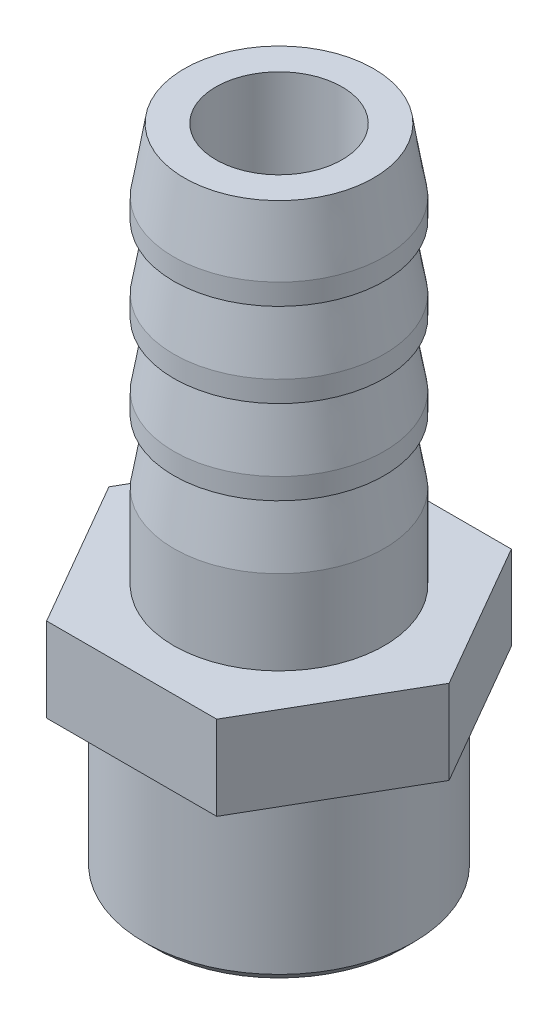
SolidWorks part; units mm, degrees
ref_plane "前视基准面" through (0, 0, 0) normal (0, 0, 1) x (1, 0, 0)
ref_plane "上视基准面" through (0, 0, 0) normal (0, 1, 0) x (1, 0, 0)
ref_plane "右视基准面" through (0, 0, 0) normal (1, 0, 0) x (0, 0, -1)
sketch "草图1" plane through (0, 0, 0) normal (0, 0, 1) x (1, 0, 0)
  line L0 (0, -266.5887) -> (0, 13062.8486) construction
  line L1 (-5, 4) -> (-4.5, 7)
  line L2 (0, 0) -> (-5, 0)
  line L3 (0, 0) -> (0, 19)
  line L5 (-5, 0) -> (-5, 4)
  line L6 (-5, 8) -> (-4.5, 11)
  line L7 (-5, 7) -> (-4.5, 7)
  line L8 (-5, 7) -> (-5, 8)
  line L11 (-4.5, -988.826) -> (-4.5, 49011.174) construction
  line L12 (-5, 11) -> (-4.5, 11)
  line L13 (-5, 11) -> (-5, 12)
  line L16 (-5, 12) -> (-4.5, 15)
  line L17 (-5, 15) -> (-4.5, 15)
  line L18 (-5, 15) -> (-5, 16)
  line L19 (-5, 16) -> (-4.5, 19)
  line L20 (-4.5, 19) -> (0, 19)
  point P9 (-5, 0.826)
  dimension "D1" = 5
  dimension "D2" = 19
  dimension "D3" = 1
  dimension "D4" = 3
  dimension "D5" = 4.5
  dimension "D6" = 1
  dimension "D7" = 3
  dimension "D8" = 3
  dimension "D9" = 1
  dimension "D10" = 3
revolve "旋转1" add sketch "草图1" angle 360 about L3
sketch "草图2" plane through (0, 0, 0) normal (0, -1, 0) x (1, 0, 0)
  line L0 (-1000, 0) -> (49000, 0) construction
  line L1 (8.0829, 0) -> (4.0415, 7)
  line L2 (4.0415, 7) -> (-4.0415, 7)
  line L3 (-4.0415, 7) -> (-8.0829, 0)
  line L4 (-8.0829, 0) -> (-4.0415, -7)
  line L5 (-4.0415, -7) -> (4.0415, -7)
  line L6 (4.0415, -7) -> (8.0829, 0)
  circle A0 centre (0, 0) radius 7 construction
  dimension "D1" = 14
extrude "凸台-拉伸1" add sketch "草图2" along normal blind 4
sketch "草图3" plane through (0, -4, 0) normal (0, -1, 0) x (1, 0, 0)
  circle A0 centre (0, 0) radius 6.4
  dimension "D1" = 12.8
extrude "凸台-拉伸2" add sketch "草图3" along normal blind 8
cosmetic thread "装饰螺纹线1" parameters "D2"=8.566
sketch "草图4" plane through (0, 19, 0) normal (0, 1, 0) x (1, 0, 0)
  circle A0 centre (0, 0) radius 3
  dimension "D1" = 6
extrude "切除-拉伸1" cut sketch "草图4" against normal up to next
chamfer "倒角1" distance 0.5 angle 45 1 edges at (6.4, -12, 0)
